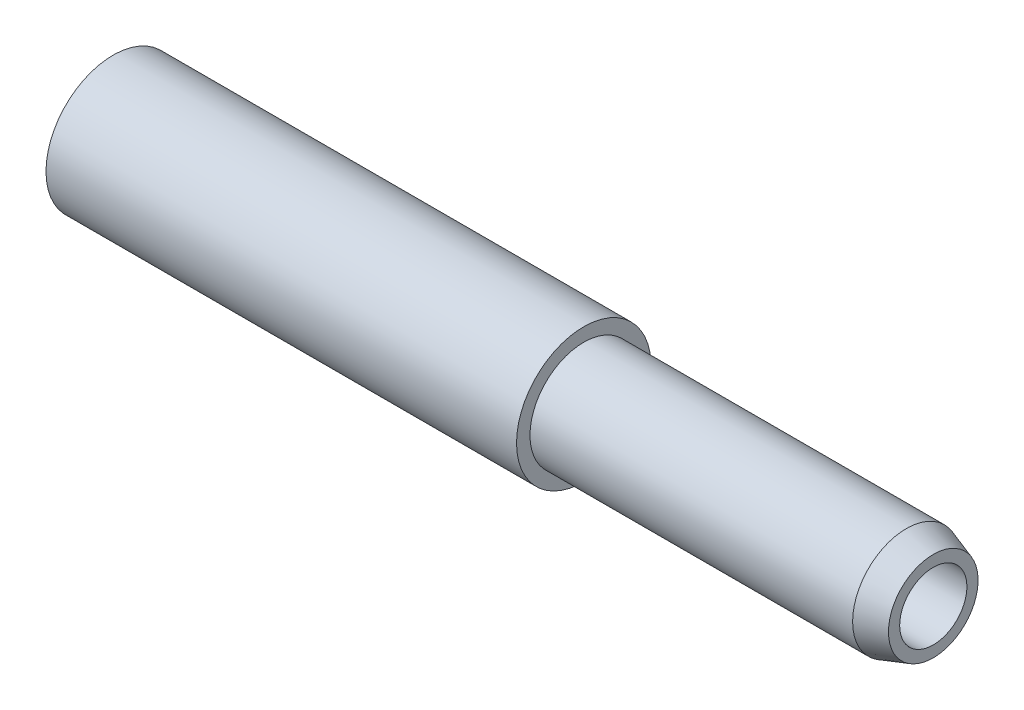
SolidWorks part; units mm, degrees
ref_plane "Front" through (0, 0, 0) normal (0, 0, 1) x (1, 0, 0)
ref_plane "Top" through (0, 0, 0) normal (0, 1, 0) x (1, 0, 0)
ref_plane "Right" through (0, 0, 0) normal (1, 0, 0) x (0, 0, -1)
sketch "Sketch1" plane through (0, 0, 0) normal (0, 0, 1) x (1, 0, 0)
  line L0 (0, 0) -> (148.5879, 0) construction
  line L1 (0, 7.5) -> (0, 15)
  line L2 (0, 7.5) -> (8, 7.5)
  line L3 (8, 7.5) -> (8, 3.25)
  line L4 (8, 3.25) -> (33, 3.25)
  line L5 (33, 3.25) -> (33, 7.5)
  line L6 (33, 7.5) -> (183, 7.5)
  line L7 (183, 12) -> (183, 7.5)
  line L9 (183, 12) -> (105, 12)
  line L10 (105, 12) -> (105, 15)
  line L11 (105, 15) -> (0, 15)
  dimension "D1" = 15
  dimension "D2" = 30
  dimension "D3" = 8
  dimension "D4" = 6.5
  dimension "D5" = 15
  dimension "D6" = 24
  dimension "D7" = 78
  dimension "D8" = 25
  dimension "D9" = 105
revolve "Revolve1" add sketch "Sketch1" angle 360 about L0
cosmetic thread "Cosmetic Thread1" [suppressed] parameters "D2"=21
chamfer "Chamfer1" distance 2 distance2 6 1 edges at (183, 0, 12)
